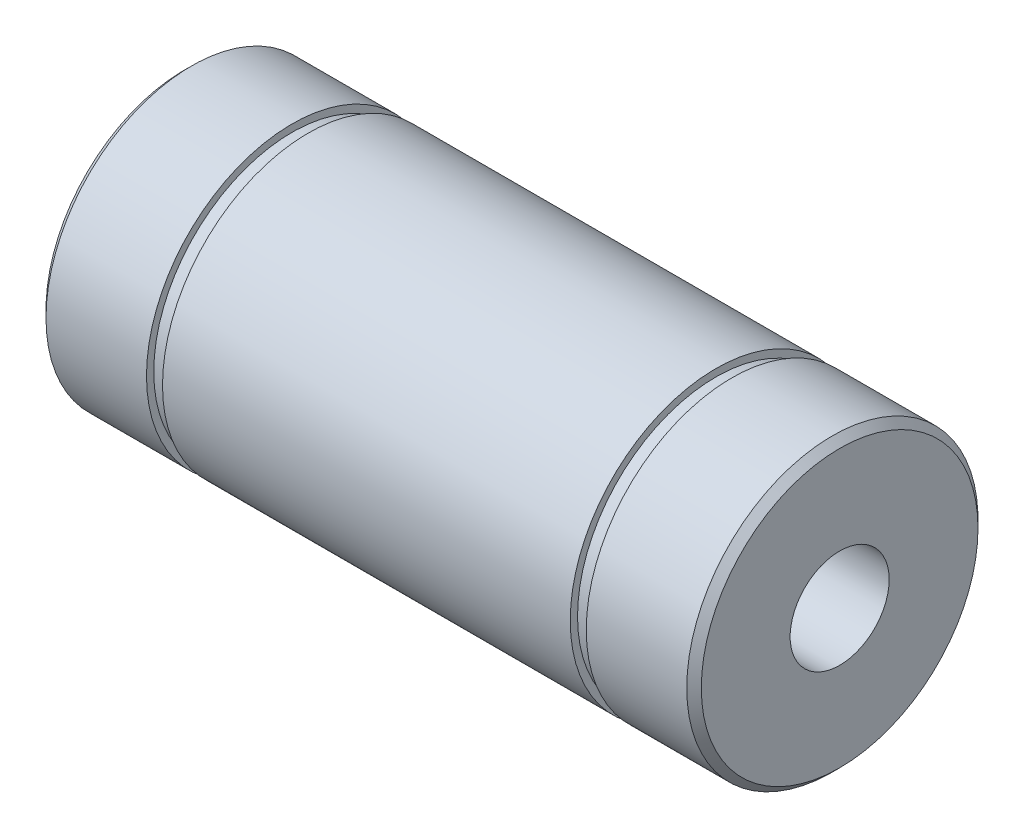
from build123d import *

# Parameters (mm, degrees)
SKETCH_1_R      = 10
EXTRUDE_1_DEPTH = 22.5
CHAMFER_1_SIZE  = 0.5
SKETCH_4_W      = 1.1
SKETCH_4_H      = 0.5


with BuildPart() as part:
    # 草图1 → 凸台-拉伸1 (new, symmetric)
    with BuildSketch(Plane(origin=(0, 0, 0), x_dir=(0, 0, -1), z_dir=(1, 0, 0))):
        with Locations(Location((0, 0, 0), (0, 0, 180))):
            Circle(SKETCH_1_R)
    extrude(amount=EXTRUDE_1_DEPTH, both=True)

    # 草图2 → M8 螺纹孔1 (revolve, cut)
    with BuildSketch(Plane(origin=(22.5, 0, 0), x_dir=(0, 0, -1), z_dir=(0, 1, 0))):
        Polygon((0, 0), (0, 21.792926105), (3.4, 19.75), (3.4, 0), align=None)
    hole_wizard_m8_1 = revolve(axis=Axis((28.85, 0, 0), (-1, 0, 0)), mode=Mode.SUBTRACT)

    # 镜向1: M8 螺纹孔1 across plane
    add(hole_wizard_m8_1.mirror(Plane(origin=(0, 0, 0), x_dir=(0, 0, 1), z_dir=(1, 0, 0))), mode=Mode.SUBTRACT)

    # 倒角1
    chamfer_1_edges = [part.edges().sort_by_distance(p)[0] for p in [
        (-22.5, 0, -10),
        (22.5, 0, -10),
    ]]
    chamfer(chamfer_1_edges, length=CHAMFER_1_SIZE)

    # 草图4 → 切除-旋转1 (revolve, cut)
    with BuildSketch(Plane.XY, mode=Mode.PRIVATE) as cut_revolve_1_sk:
        with Locations((-14.55, 9.75)):
            Rectangle(SKETCH_4_W, SKETCH_4_H)
    cut_revolve_1 = revolve(cut_revolve_1_sk.sketch.rotate(Axis((0, 0, 0), (1, 0, 0)), 90), axis=Axis((0, 0, 0), (1, 0, 0)), mode=Mode.SUBTRACT)

    # 镜向2: 切除-旋转1 across plane
    add(cut_revolve_1.mirror(Plane(origin=(0, 0, 0), x_dir=(0, 0, 1), z_dir=(1, 0, 0))), mode=Mode.SUBTRACT)


solid = part.part
